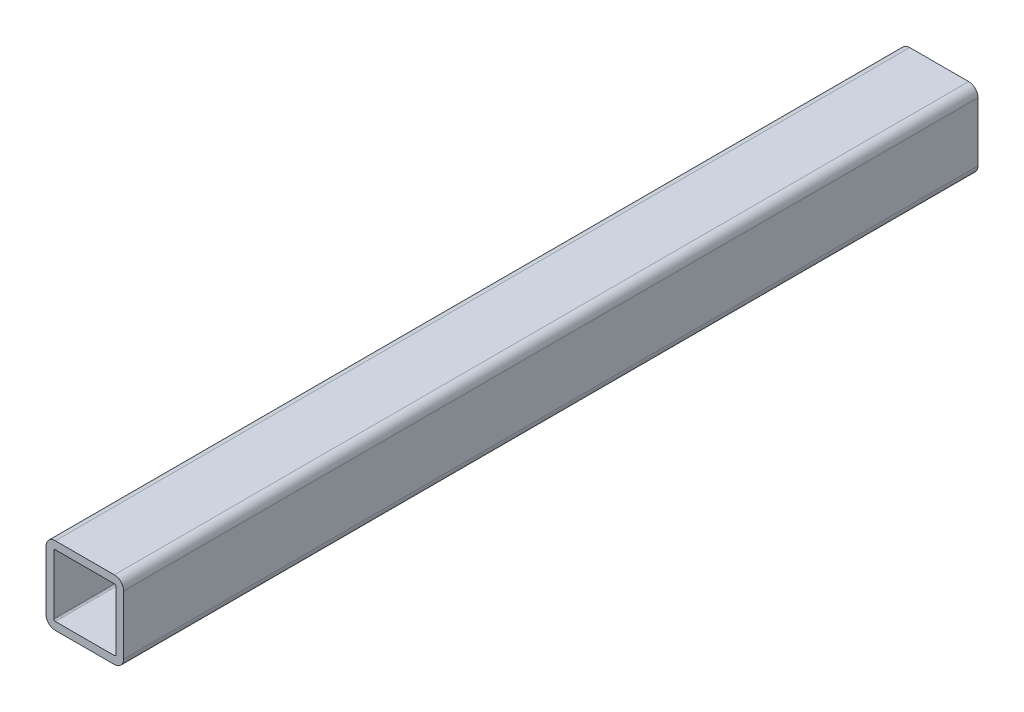
from build123d import *

# Parameters (mm, degrees)
BOSS_EXTRUDE1_DEPTH = 550


with BuildPart() as part:
    # Sketch1 → Boss-Extrude1 (new body)
    with BuildSketch(Plane.XY):
        with BuildLine():
            Line((6, 0), (44, 0))
            ThreePointArc((44, 0), (48.242640687, 1.757359313), (50, 6))
            Line((50, 6), (50, 44))
            ThreePointArc((50, 44), (48.242640687, 48.242640687), (44, 50))
            Line((44, 50), (6, 50))
            ThreePointArc((6, 50), (1.757359313, 48.242640687), (0, 44))
            Line((0, 44), (0, 6))
            ThreePointArc((0, 6), (1.757359313, 1.757359313), (6, 0))
        make_face()
        with BuildLine():
            Line((6, 45), (44, 45))
            ThreePointArc((44, 45), (44.707106781, 44.707106781), (45, 44))
            Line((45, 44), (45, 6))
            ThreePointArc((45, 6), (44.707106781, 5.292893219), (44, 5))
            Line((44, 5), (6, 5))
            ThreePointArc((6, 5), (5.292893219, 5.292893219), (5, 6))
            Line((5, 6), (5, 44))
            ThreePointArc((5, 44), (5.292893219, 44.707106781), (6, 45))
        make_face(mode=Mode.SUBTRACT)
    extrude(amount=BOSS_EXTRUDE1_DEPTH)


solid = part.part
